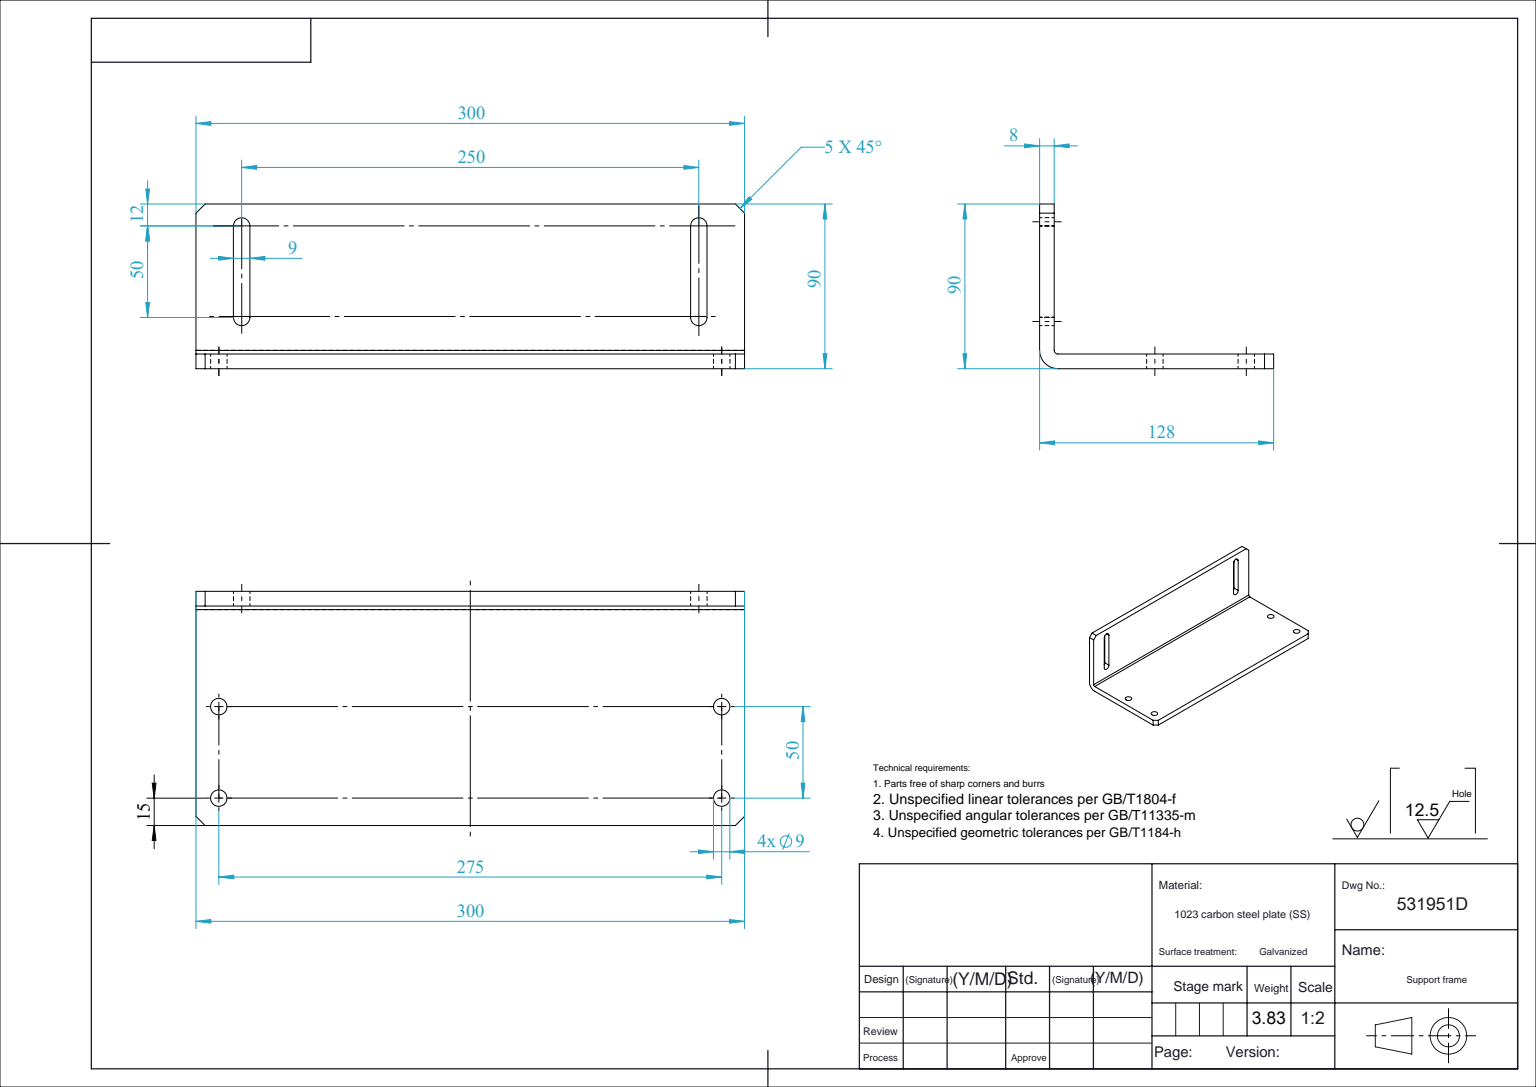
from build123d import *

# Parameters (mm, degrees)
BOSS_EXTRUDE1_DEPTH = 300
SKETCH2_R           = 4.5
CUT_EXTRUDE1_DEPTH  = 300
CUT_EXTRUDE2_DEPTH  = 300
CHAMFER1_SIZE       = 5
FILLET1_R           = 2
FILLET2_R           = 10


with BuildPart() as part:
    # Sketch1 → Boss-Extrude1 (new body)
    with BuildSketch(Plane.XY):
        Polygon((0, 0), (0, -90), (128, -90), (128, -82), (8, -82), (8, 0), align=None)
    extrude(amount=BOSS_EXTRUDE1_DEPTH)

    # Sketch2 → Cut-Extrude1 (cut)
    with BuildSketch(Plane(origin=(0, -82, 0), x_dir=(1, 0, 0), z_dir=(0, 1, 0))):
        with Locations(Location((63, -12.5, 0), (0, 0, 270))):
            Circle(SKETCH2_R)
        with Locations(Location((113, -12.5, 0), (0, 0, 270))):
            Circle(SKETCH2_R)
        with Locations(Location((63, -287.5, 0), (0, 0, 270))):
            Circle(SKETCH2_R)
        with Locations(Location((113, -287.5, 0), (0, 0, 270))):
            Circle(SKETCH2_R)
    extrude(amount=-CUT_EXTRUDE1_DEPTH, mode=Mode.SUBTRACT)

    # Sketch3 → Cut-Extrude2 (cut)
    with BuildSketch(Plane(origin=(8, 0, 0), x_dir=(0, 0, -1), z_dir=(1, 0, 0))):
        with BuildLine():
            Line((-270.5, -12), (-270.5, -62))
            ThreePointArc((-270.5, -62), (-275, -66.5), (-279.5, -62))
            Line((-279.5, -62), (-279.5, -12))
            ThreePointArc((-279.5, -12), (-275, -7.5), (-270.5, -12))
        make_face()
        with BuildLine():
            Line((-29.5, -12), (-29.5, -62))
            ThreePointArc((-29.5, -62), (-25, -66.5), (-20.5, -62))
            Line((-20.5, -62), (-20.5, -12))
            ThreePointArc((-20.5, -12), (-25, -7.5), (-29.5, -12))
        make_face()
    extrude(amount=-CUT_EXTRUDE2_DEPTH, mode=Mode.SUBTRACT)

    # Chamfer1
    chamfer1_edges = [part.edges().sort_by_distance(p)[0] for p in [
        (4, 0, 300),
        (4, 0, 0),
        (128, -86, 0),
        (128, -86, 300),
    ]]
    chamfer(chamfer1_edges, length=CHAMFER1_SIZE)

    # Fillet1
    fillet1_edges = [part.edges().sort_by_distance(p)[0] for p in [
        (8, -82, 150),
    ]]
    fillet(fillet1_edges, radius=FILLET1_R)

    # Fillet2
    fillet2_edges = [part.edges().sort_by_distance(p)[0] for p in [
        (0, -90, 150),
    ]]
    fillet(fillet2_edges, radius=FILLET2_R)


solid = part.part
